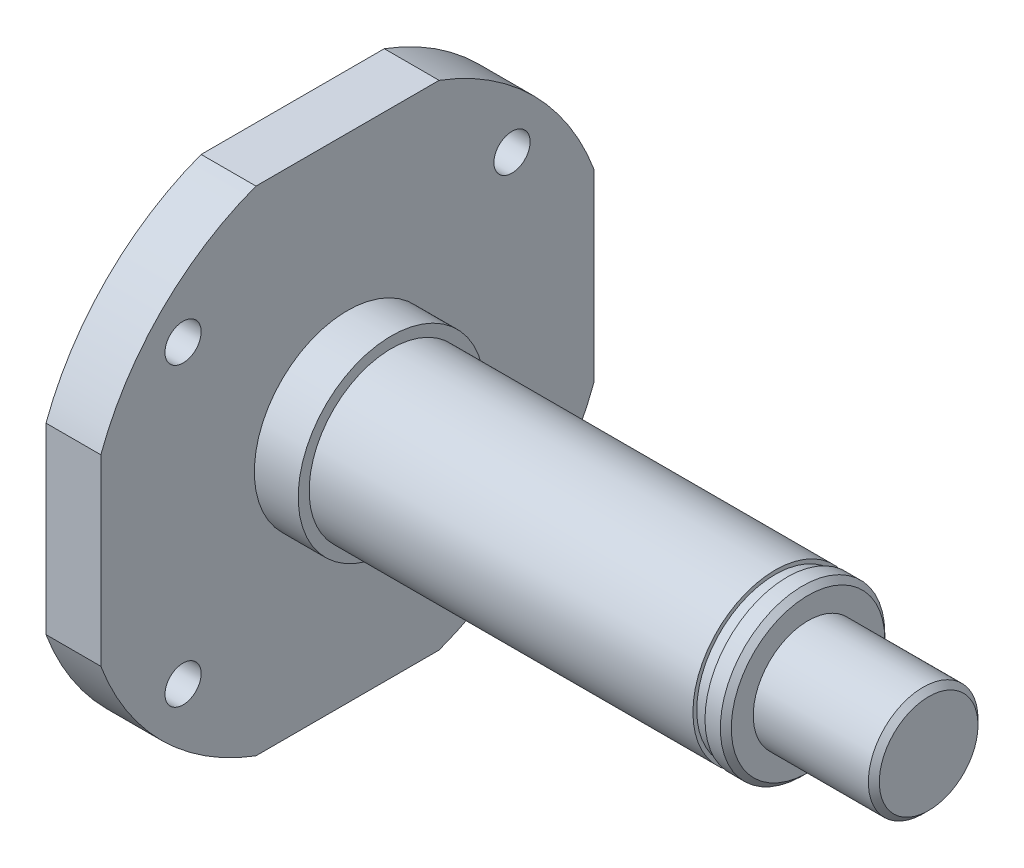
SolidWorks part; units mm, degrees
material "6061 合金"
ref_plane "前视" through (0, 0, 0) normal (0, 0, 1) x (1, 0, 0)
ref_plane "上视" through (0, 0, 0) normal (0, 1, 0) x (1, 0, 0)
ref_plane "右视" through (0, 0, 0) normal (1, 0, 0) x (0, 0, -1)
sketch "草图1" plane through (0, 0, 0) normal (0, 1, 0) x (1, 0, 0)
  line L0 (0, 0) -> (0, 24)
  line L1 (0, 24) -> (5, 24)
  line L2 (5, 24) -> (5, 8.5)
  line L3 (5, 8.5) -> (9, 8.5)
  line L4 (9, 8.5) -> (9, 7.5)
  line L5 (9, 7.5) -> (47, 7.5)
  line L6 (47, 7.5) -> (47, 5)
  line L7 (47, 5) -> (58, 5)
  line L8 (58, 5) -> (58, 0)
  line L9 (58, 0) -> (0, 0)
  line L10 (0, 0) -> (75.0357, 0) construction
  dimension "D1" = 48
  dimension "D2" = 5
  dimension "D3" = 17
  dimension "D4" = 15
  dimension "D5" = 4
  dimension "D6" = 38
  dimension "D7" = 10
  dimension "D8" = 11
revolve "旋转1" add sketch "草图1" angle 360 about L9
sketch "草图2" plane through (0, 0, 0) normal (-1, 0, 0) x (0, 0, 1)
  line L1 (-15, -13.5) -> (15, -13.5)
  line L2 (-15, -13.5) -> (-15, 13.5)
  line L3 (-15, 13.5) -> (15, 13.5)
  line L4 (15, -13.5) -> (15, 13.5)
  line L5 (-15, -13.5) -> (15, 13.5) construction
  line L6 (-15, 13.5) -> (15, -13.5) construction
  point P0 (0, 0)
  dimension "D1" = 30
  dimension "D2" = 27
hole_wizard "M4 螺纹孔1" positions "3D草图1" profile "草图3" tap size "M4" standard "GB" end condition through all
sketch3d "3D草图1"
  point P0 (0, 13.5, -15)
  point P3 (0, 13.5, 15)
  point P6 (0, -13.5, -15)
  point P9 (0, -13.5, 15)
sketch "草图3" plane through (0, 13.5, -15) normal (0, 1, 0) x (0, 0, 1)
  line L0 (0, 0) -> (0, 58)
  line L1 (0, 58) -> (1.65, 58)
  line L2 (1.65, 58) -> (1.65, 0)
  line L5 (1.65, 0) -> (0, 0)
  line L11 (0, -6.35) -> (0, 107.95) construction
  dimension "通孔螺纹孔钻头直径" = 3.3
  dimension "通孔螺纹孔钻头深度" = 58
cosmetic thread "孔螺蚊线1" parameters "D2"=4
cosmetic thread "孔螺蚊线2" parameters "D2"=4
cosmetic thread "孔螺蚊线3" parameters "D2"=4
cosmetic thread "孔螺蚊线4" parameters "D2"=4
sketch "草图4" plane through (0, 0, 0) normal (-1, 0, 0) x (0, 0, 1)
  line L1 (-22.5, -22.5) -> (22.5, -22.5)
  line L2 (-22.5, -22.5) -> (-22.5, 22.5)
  line L3 (-22.5, 22.5) -> (22.5, 22.5)
  line L4 (22.5, -22.5) -> (22.5, 22.5)
  line L5 (-22.5, -22.5) -> (22.5, 22.5) construction
  line L6 (-22.5, 22.5) -> (22.5, -22.5) construction
  point P0 (0, 0)
  dimension "D1" = 45
  dimension "D2" = 45
extrude "切除-拉伸1" cut sketch "草图4" against normal blind 10 flip side to cut
chamfer "倒角1" distance 0.5 angle 45 2 edges at (47, 0, -7.5) (58, 0, -5)
sketch "草图5" plane through (0, 0, 0) normal (0, 1, 0) x (1, 0, 0)
  line L0 (0, 0) -> (33.0216, 0) construction
  line L1 (46.5, 7.5) -> (9, 7.5) construction
  line L2 (44, 7.5) -> (45.1, 7.5)
  line L3 (44, 7.5) -> (44, 7.15)
  line L4 (44, 7.15) -> (45.1, 7.15)
  line L5 (45.1, 7.5) -> (45.1, 7.15)
  line L6 (9, -8.5) -> (9, 8.5) construction
  dimension "D1" = 14.3
  dimension "D2" = 1.1
  dimension "D3" = 35
revolve "切除-旋转1" cut sketch "草图5" angle 360 about L0
